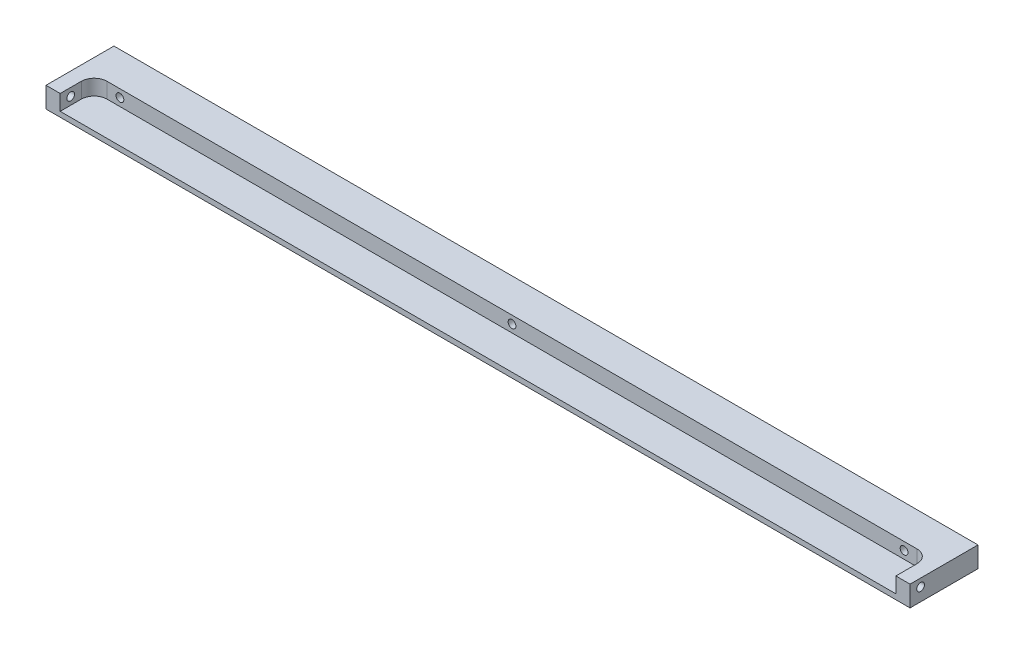
SolidWorks part; units mm, degrees
ref_plane "Front Plane" through (0, 0, 0) normal (0, 0, 1) x (1, 0, 0)
ref_plane "Top Plane" through (0, 0, 0) normal (0, 1, 0) x (1, 0, 0)
ref_plane "Right Plane" through (0, 0, 0) normal (1, 0, 0) x (0, 0, -1)
sketch "Sketch1" plane through (0, 0, 0) normal (0, 1, 0) x (1, 0, 0)
  line L1 (335, 26.3427) -> (-335, 26.3427)
  line L2 (335, 26.3427) -> (335, -26.3427)
  line L3 (335, -26.3427) -> (-335, -26.3427)
  line L4 (-335, 26.3427) -> (-335, -26.3427)
  line L5 (335, 26.3427) -> (-335, -26.3427) construction
  line L6 (335, -26.3427) -> (-335, 26.3427) construction
  point P0 (0, 0)
  dimension "D1" = 670
extrude "Boss-Extrude1" add sketch "Sketch1" along normal blind 16
sketch "Sketch3" plane through (0, 16, 0) normal (0, 1, 0) x (1, 0, 0)
  line L0 (-335, 26.3427) -> (-335, -26.3427) construction
  line L1 (-324, 0) -> (324, 0)
  line L2 (-324, 0) -> (-324, -81.0225)
  line L3 (-324, -81.0225) -> (324, -81.0225)
  line L4 (324, 0) -> (324, -81.0225)
  line L5 (335, -26.3427) -> (335, 26.3427) construction
  dimension "D1" = 11
  dimension "D2" = 11
extrude "Cut-Extrude2" cut sketch "Sketch3" against normal blind 12
fillet "Fillet1" radius 10 2 edges at (324, 10, 0) (-324, 10, 0)
sketch "Sketch5" plane through (324, 0, 0) normal (-1, 0, 0) x (0, 0, 1)
  line L0 (10, 4) -> (26.3427, 16) construction
  line L1 (10, 16) -> (26.3427, 4) construction
hole_wizard "Ø6.0mm Dowel Hole1" positions "Sketch8" profile "Sketch10" hole size "Ø6.0" standard "ANSI Metric"
sketch "Sketch8" plane through (324, 0, 0) normal (-1, 0, 0) x (0, 0, 1)
  line L0 (10, 4) -> (26.3427, 16) construction
  point P0 (18.1714, 10)
  point P3 (18.1844, 9.8865)
  point P4 (23.2254, 8.7237)
  point P7 (18.1714, 10)
sketch "Sketch10" plane through (324, 10, 18.1714) normal (0, 1, 0) x (0, 0, 1)
  line L0 (0, 0) -> (0, 11)
  line L1 (0, 11) -> (3, 11)
  line L2 (3, 11) -> (3, 0)
  line L5 (3, 0) -> (0, 0)
  line L11 (0, -6.35) -> (0, 107.95) construction
  dimension "Thru Hole Dia." = 6
  dimension "Thru Hole Depth" = 11
mirror "Mirror1" about plane through (0, 0, 0) normal (1, 0, 0) of "Ø6.0mm Dowel Hole1"
sketch "Sketch11" plane through (0, 0, 0) normal (0, 0, 1) x (1, 0, 0)
  line L0 (314, 10) -> (-314, 10) construction
  line L1 (314, 4) -> (314, 16) construction
  line L2 (-314, 16) -> (-314, 4) construction
  circle A0 centre (304, 10) radius 3
  point P8 (0, 0)
  point P9 (0, 0)
  dimension "D1" = 6
  dimension "D2" = 10
hole_wizard "Ø6.0mm Dowel Hole2" positions "Sketch12" profile "Sketch13" hole size "Ø6.0" standard "ANSI Metric" end condition through all
sketch "Sketch12" plane through (0, 0, 0) normal (0, 0, 1) x (1, 0, 0)
  point P0 (304, 10)
  point P4 (0, 10)
sketch "Sketch13" plane through (304, 10, 0) normal (1, 0, 0) x (0, -1, 0)
  line L0 (0, 0) -> (0, 26.3427)
  line L1 (0, 26.3427) -> (3, 26.3427)
  line L2 (3, 26.3427) -> (3, 0)
  line L5 (3, 0) -> (0, 0)
  line L11 (0, -6.35) -> (0, 107.95) construction
  dimension "Thru Hole Dia." = 6
  dimension "Thru Hole Depth" = 26.3427
mirror "Mirror2" about plane through (0, 0, 0) normal (1, 0, 0) of "Ø6.0mm Dowel Hole2"
sketch "Sketch14" plane through (0, 16, 0) normal (0, 1, 0) x (1, 0, 0)
  line L1 (335, 26.3427) -> (-335, 26.3427) construction
  circle A0 centre (0, 27.8427) radius 1.5
  point P4 (0, 0)
  dimension "D1" = 3
